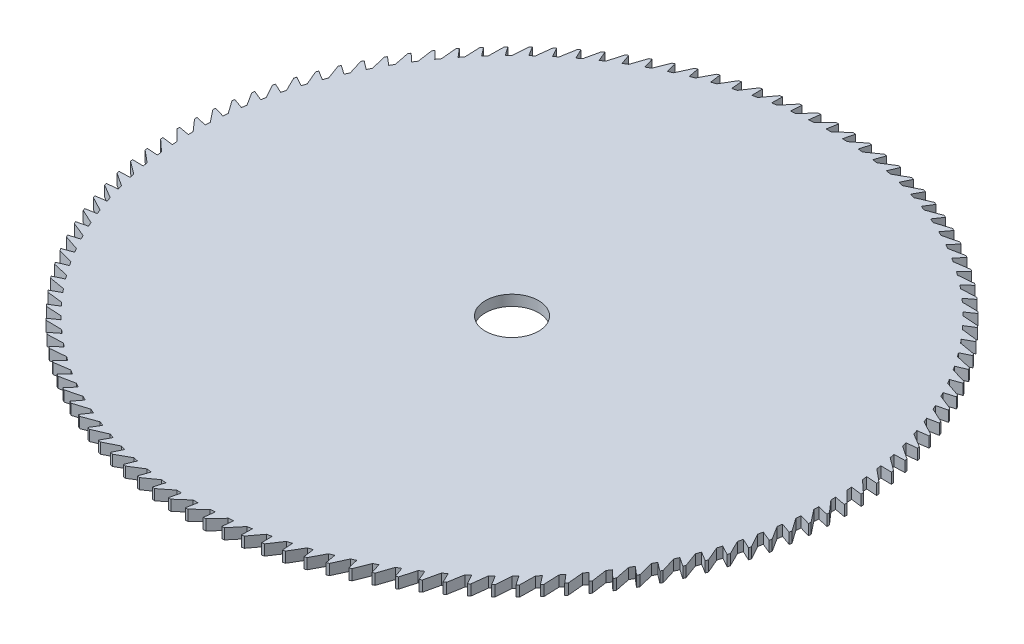
from build123d import *

# Parameters (mm, degrees)
SKETCH2_R           = 150
SKETCH2_R_2         = 12.5
BOSS_EXTRUDE1_DEPTH = 5
BOSS_EXTRUDE2_DEPTH = 5


with BuildPart() as part:
    # Sketch2 → Boss-Extrude1 (new body)
    with BuildSketch(Plane(origin=(0, 0, 0), x_dir=(1, 0, 0), z_dir=(0, 1, 0))):
        with Locations(Location((0, 0, 0), (0, 0, 270))):
            Circle(SKETCH2_R)
        with Locations(Location((0, 0, 0), (0, 0, 270))):
            Circle(SKETCH2_R_2, mode=Mode.SUBTRACT)
    extrude(amount=BOSS_EXTRUDE1_DEPTH)

    # Sketch3 → Boss-Extrude2 (add)
    with BuildSketch(Plane(origin=(0, 5, 0), x_dir=(1, 0, 0), z_dir=(0, 1, 0))):
        with BuildLine():
            Line((0, 150), (5.590008371, 154.899166578))
            ThreePointArc((5.590008371, 154.899166578), (6.178302205, 154.876817445), (6.76650691, 154.85223403))
            Line((6.76650691, 154.85223403), (5.590008371, 149.895803165))
            ThreePointArc((5.590008371, 149.895803165), (2.795489696, 149.973948529), (0, 150))
        make_face()
        with BuildLine():
            Line((7.850393436, 149.794430213), (13.689143463, 154.39432422))
            ThreePointArc((13.689143463, 154.39432422), (14.275461398, 154.341216795), (14.861573392, 154.285882816))
            Line((14.861573392, 154.285882816), (13.427287654, 149.397817743))
            ThreePointArc((13.427287654, 149.397817743), (10.640688583, 149.622109818), (7.850393436, 149.794430213))
        make_face()
        with BuildLine():
            Line((15.67926949, 149.178284305), (21.750757564, 153.466297751))
            ThreePointArc((21.750757564, 153.466297751), (22.333492543, 153.382577599), (22.915905334, 153.296644721))
            Line((22.915905334, 153.296644721), (21.227763675, 148.490343286))
            ThreePointArc((21.227763675, 148.490343286), (18.456722081, 148.860167305), (15.67926949, 149.178284305))
        make_face()
        with BuildLine():
            Line((23.465169756, 148.153251089), (29.752754351, 152.117630827))
            ThreePointArc((29.752754351, 152.117630827), (30.330309137, 152.003527418), (30.907426372, 151.887231178))
            Line((30.907426372, 151.887231178), (28.970055872, 147.175867121))
            ThreePointArc((28.970055872, 147.175867121), (26.222166987, 147.69020942), (23.465169756, 148.153251089))
        make_face()
        with BuildLine():
            Line((31.186753623, 146.72214011), (37.673200906, 150.352020051))
            ThreePointArc((37.673200906, 150.352020051), (38.243992462, 150.207846135), (38.814232304, 150.061505293))
            Line((38.814232304, 150.061505293), (36.632943159, 145.457992134))
            ThreePointArc((36.632943159, 145.457992134), (33.915738757, 146.115442937), (31.186753623, 146.72214011))
        make_face()
        with BuildLine():
            Line((38.822856765, 144.888873943), (45.490387836, 148.174304839))
            ThreePointArc((45.490387836, 148.174304839), (46.052851662, 148.000455586), (46.614651122, 147.824471251))
            Line((46.614651122, 147.824471251), (44.195422095, 143.3414269))
            ThreePointArc((44.195422095, 143.3414269), (41.516349843, 144.140184181), (38.822856765, 144.888873943))
        make_face()
        with BuildLine():
            Line((46.352549156, 142.658477444), (53.182888775, 145.590454157))
            ThreePointArc((53.182888775, 145.590454157), (53.735483197, 145.387406076), (54.287302422, 145.18226061))
            Line((54.287302422, 145.18226061), (51.636764451, 140.83197278))
            ThreePointArc((51.636764451, 140.83197278), (49.003167501, 141.769847199), (46.352549156, 142.658477444))
        make_face()
        with BuildLine():
            Line((53.755192432, 140.037063975), (60.729619112, 142.60755016))
            ThreePointArc((60.729619112, 142.60755016), (61.270829508, 142.375859792), (61.811155999, 142.142115483))
            Line((61.811155999, 142.142115483), (58.936574025, 137.936508011))
            ThreePointArc((58.936574025, 137.936508011), (56.355670883, 139.010928921), (53.755192432, 140.037063975))
        make_face()
        with BuildLine():
            Line((61.010496461, 137.031818646), (68.109893785, 139.23376878))
            ThreePointArc((68.109893785, 139.23376878), (68.638236733, 138.974071172), (69.165589494, 138.712368698))
            Line((69.165589494, 138.712368698), (66.074842546, 134.662968861))
            ThreePointArc((66.074842546, 134.662968861), (63.553707287, 135.870991348), (61.010496461, 137.031818646))
        make_face()
        with BuildLine():
            Line((68.098574961, 133.650978628), (75.303483973, 135.478357318))
            ThreePointArc((75.303483973, 135.478357318), (75.817511323, 135.191364283), (76.330444916, 134.902420953))
            Line((76.330444916, 134.902420953), (73.032004517, 131.020327874))
            ThreePointArc((73.032004517, 131.020327874), (70.577547398, 132.358640833), (68.098574961, 133.650978628))
        make_face()
        with BuildLine():
            Line((75, 129.903810568), (82.290672546, 131.351609096))
            ThreePointArc((82.290672546, 131.351609096), (82.788975384, 131.038107262), (83.286083894, 130.722715048))
            Line((83.286083894, 130.722715048), (79.788990839, 127.018569276))
            ThreePointArc((79.788990839, 127.018569276), (77.407939358, 128.483504484), (75, 129.903810568))
        make_face()
        with BuildLine():
            Line((81.695855252, 125.800585192), (89.052308105, 126.864835243))
            ThreePointArc((89.052308105, 126.864835243), (89.533520619, 126.525683897), (90.013441506, 126.184707268))
            Line((90.013441506, 126.184707268), (86.327281084, 122.668661608))
            ThreePointArc((86.327281084, 122.668661608), (84.026161536, 124.256203779), (81.695855252, 125.800585192))
        make_face()
        with BuildLine():
            Line((88.167787844, 121.352549156), (95.569857478, 122.030333695))
            ThreePointArc((95.569857478, 122.030333695), (96.032660697, 121.666462427), (96.49407853, 121.300835976))
            Line((96.49407853, 121.300835976), (92.628954252, 117.982527665))
            ThreePointArc((92.628954252, 117.982527665), (90.414073845, 119.688325457), (88.167787844, 121.352549156))
        make_face()
        with BuildLine():
            Line((94.398058657, 116.571894219), (101.825456514, 116.861355485))
            ThreePointArc((101.825456514, 116.861355485), (102.268581926, 116.473761641), (102.710231993, 116.084487525))
            Line((102.710231993, 116.084487525), (98.676737895, 112.973011815))
            ThreePointArc((98.676737895, 112.973011815), (96.554167463, 114.792389754), (94.398058657, 116.571894219))
        make_face()
        with BuildLine():
            Line((100.369590954, 111.471723822), (107.801959052, 111.372068422))
            ThreePointArc((107.801959052, 111.372068422), (108.224192082, 110.96181437), (108.64486385, 110.549959562))
            Line((108.64486385, 110.549959562), (104.454055458, 107.653844792))
            ThreePointArc((104.454055458, 107.653844792), (102.42961282, 109.58181609), (100.369590954, 111.471723822))
        make_face()
        with BuildLine():
            Line((106.066017178, 106.066017178), (113.482983913, 105.577518261))
            ThreePointArc((113.482983913, 105.577518261), (113.883167249, 105.145728478), (114.281707686, 104.712421844))
            Line((114.281707686, 104.712421844), (109.945071715, 102.039606063))
            ThreePointArc((109.945071715, 102.039606063), (108.024305727, 104.070886285), (106.066017178, 106.066017178))
        make_face()
        with BuildLine():
            Line((111.471723822, 100.369590954), (118.852959804, 99.493587461))
            ThreePointArc((118.852959804, 99.493587461), (119.229996571, 99.041445454), (119.605313305, 98.587874656))
            Line((119.605313305, 98.587874656), (115.134736174, 96.145683867))
            ThreePointArc((115.134736174, 96.145683867), (113.322911521, 98.274705415), (111.471723822, 100.369590954))
        make_face()
        with BuildLine():
            Line((116.571894219, 94.398058657), (123.897167993, 93.136951654))
            ThreePointArc((123.897167993, 93.136951654), (124.25002476, 92.665696711), (124.601089074, 92.193104957))
            Line((124.601089074, 92.193104957), (120.008824323, 89.988233034))
            ThreePointArc((120.008824323, 89.988233034), (118.310907092, 92.209160408), (116.571894219, 94.398058657))
        make_face()
        with BuildLine():
            Line((121.352549156, 88.167787844), (128.601782656, 86.525033936))
            ThreePointArc((128.601782656, 86.525033936), (128.929492268, 86.035957736), (129.255341919, 85.545640365))
            Line((129.255341919, 85.545640365), (124.553976627, 83.58413071))
            ThreePointArc((124.553976627, 83.58413071), (122.97462069, 85.890876501), (121.352549156, 88.167787844))
        make_face()
        with BuildLine():
            Line((125.800585192, 81.695855252), (132.953908773, 79.675957114))
            ThreePointArc((132.953908773, 79.675957114), (133.255572999, 79.17040018), (133.555314856, 78.663701119))
            Line((133.555314856, 78.663701119), (128.757735138, 76.950930093))
            ThreePointArc((128.757735138, 76.950930093), (127.3012694, 79.337171673), (125.800585192, 81.695855252))
        make_face()
        with BuildLine():
            Line((129.903810568, 75), (136.941617467, 72.608494032))
            ThreePointArc((136.941617467, 72.608494032), (137.216409467, 72.08784206), (137.489221958, 71.566150136))
            Line((137.489221958, 71.566150136), (132.608577647, 70.106812326))
            ThreePointArc((132.608577647, 70.106812326), (131.27899418, 72.566009171), (129.903810568, 75))
        make_face()
        with BuildLine():
            Line((133.650978628, 68.098574961), (140.553978706, 65.342016115))
            ThreePointArc((140.553978706, 65.342016115), (140.801145295, 64.807696177), (141.04628066, 64.27244131))
            Line((141.04628066, 64.27244131), (136.095949262, 63.070536659))
            ThreePointArc((136.095949262, 63.070536659), (134.896892362, 65.595948283), (133.650978628, 68.098574961))
        make_face()
        with BuildLine():
            Line((137.031818646, 61.010496461), (143.781091259, 57.896440273))
            ThreePointArc((143.781091259, 57.896440273), (143.99995497, 57.349916902), (144.21674131, 56.802566191))
            Line((144.21674131, 56.802566191), (139.210291341, 55.861389035))
            ThreePointArc((139.210291341, 55.861389035), (138.145047538, 58.446093459), (137.031818646, 61.010496461))
        make_face()
        with BuildLine():
            Line((140.037063975, 53.755192432), (146.614109835, 50.292174313))
            ThreePointArc((146.614109835, 50.292174313), (146.804070778, 49.734945492), (146.991913897, 49.176999185))
            Line((146.991913897, 49.176999185), (141.943067687, 48.499129226))
            ThreePointArc((141.943067687, 48.499129226), (141.014556742, 51.136041957), (140.037063975, 53.755192432))
        make_face()
        with BuildLine():
            Line((142.658477444, 46.352549156), (149.045269328, 42.550060999))
            ThreePointArc((149.045269328, 42.550060999), (149.205806832, 41.983654053), (149.364191865, 41.416641443))
            Line((149.364191865, 41.416641443), (144.286787951, 41.003936676))
            ThreePointArc((144.286787951, 41.003936676), (143.497554847, 43.685830117), (142.658477444, 46.352549156))
        make_face()
        with BuildLine():
            Line((144.888873943, 38.822856765), (151.067906097, 34.691320926))
            ThreePointArc((151.067906097, 34.691320926), (151.198580141, 34.117288337), (151.327072966, 33.542763566))
            Line((151.327072966, 33.542763566), (146.235028158, 33.396355185))
            ThreePointArc((146.235028158, 33.396355185), (145.587236128, 36.115878454), (144.888873943, 38.822856765))
        make_face()
        with BuildLine():
            Line((146.72214011, 31.186753623), (152.676476236, 26.737494353))
            ThreePointArc((152.676476236, 26.737494353), (152.776928651, 26.157409505), (152.875177078, 25.576947305))
            Line((152.875177078, 25.576947305), (147.782448318, 25.697236606))
            ThreePointArc((147.782448318, 25.697236606), (147.277872916, 28.446935678), (146.72214011, 31.186753623))
        make_face()
        with BuildLine():
            Line((148.153251089, 23.465169756), (153.866570766, 18.710382167))
            ThreePointArc((153.866570766, 18.710382167), (153.936526219, 18.125835031), (154.004260956, 17.541026409))
            Line((154.004260956, 17.541026409), (148.924807059, 17.927683688))
            ThreePointArc((148.924807059, 17.927683688), (148.56483129, 20.700021829), (148.153251089, 23.465169756))
        make_face()
        with BuildLine():
            Line((149.178284305, 15.67926949), (154.63492772, 10.631986123))
            ThreePointArc((154.63492772, 10.631986123), (154.674194469, 10.044578904), (154.711229859, 9.45702678))
            Line((154.711229859, 9.45702678), (149.658973256, 10.108992235))
            ThreePointArc((149.658973256, 10.108992235), (149.444583789, 12.896370659), (149.178284305, 15.67926949))
        make_face()
        with BuildLine():
            Line((149.794430213, 7.850393436), (154.979441087, 2.524448545))
            ThreePointArc((154.979441087, 2.524448545), (154.987911503, 1.935791284), (154.994146035, 1.347106097))
            Line((154.994146035, 1.347106097), (149.98293461, 2.262592736))
            ThreePointArc((149.98293461, 2.262592736), (149.914719071, 5.057371433), (149.794430213, 7.850393436))
        make_face()
        with BuildLine():
            Line((150, 0), (154.899166578, -5.590008371))
            ThreePointArc((154.899166578, -5.590008371), (154.876817445, -6.178302205), (154.85223403, -6.76650691))
            Line((154.85223403, -6.76650691), (149.895803165, -5.590008371))
            ThreePointArc((149.895803165, -5.590008371), (149.973948529, -2.795489696), (150, 0))
        make_face()
        with BuildLine():
            Line((149.794430213, -7.850393436), (154.39432422, -13.689143463))
            ThreePointArc((154.39432422, -13.689143463), (154.341216795, -14.275461398), (154.285882816, -14.861573392))
            Line((154.285882816, -14.861573392), (149.397817743, -13.427287654))
            ThreePointArc((149.397817743, -13.427287654), (149.622109818, -10.640688583), (149.794430213, -7.850393436))
        make_face()
        with BuildLine():
            Line((149.178284305, -15.67926949), (153.466297751, -21.750757564))
            ThreePointArc((153.466297751, -21.750757564), (153.382577599, -22.333492543), (153.296644721, -22.915905334))
            Line((153.296644721, -22.915905334), (148.490343286, -21.227763675))
            ThreePointArc((148.490343286, -21.227763675), (148.860167305, -18.456722081), (149.178284305, -15.67926949))
        make_face()
        with BuildLine():
            Line((148.153251089, -23.465169756), (152.117630827, -29.752754351))
            ThreePointArc((152.117630827, -29.752754351), (152.003527418, -30.330309137), (151.887231178, -30.907426372))
            Line((151.887231178, -30.907426372), (147.175867121, -28.970055872))
            ThreePointArc((147.175867121, -28.970055872), (147.69020942, -26.222166987), (148.153251089, -23.465169756))
        make_face()
        with BuildLine():
            Line((146.72214011, -31.186753623), (150.352020051, -37.673200906))
            ThreePointArc((150.352020051, -37.673200906), (150.207846135, -38.243992462), (150.061505293, -38.814232304))
            Line((150.061505293, -38.814232304), (145.457992134, -36.632943159))
            ThreePointArc((145.457992134, -36.632943159), (146.115442937, -33.915738757), (146.72214011, -31.186753623))
        make_face()
        with BuildLine():
            Line((144.888873943, -38.822856765), (148.174304839, -45.490387836))
            ThreePointArc((148.174304839, -45.490387836), (148.000455586, -46.052851662), (147.824471251, -46.614651122))
            Line((147.824471251, -46.614651122), (143.3414269, -44.195422095))
            ThreePointArc((143.3414269, -44.195422095), (144.140184181, -41.516349843), (144.888873943, -38.822856765))
        make_face()
        with BuildLine():
            Line((142.658477444, -46.352549156), (145.590454157, -53.182888775))
            ThreePointArc((145.590454157, -53.182888775), (145.387406076, -53.735483197), (145.18226061, -54.287302422))
            Line((145.18226061, -54.287302422), (140.83197278, -51.636764451))
            ThreePointArc((140.83197278, -51.636764451), (141.769847199, -49.003167501), (142.658477444, -46.352549156))
        make_face()
        with BuildLine():
            Line((140.037063975, -53.755192432), (142.60755016, -60.729619112))
            ThreePointArc((142.60755016, -60.729619112), (142.375859792, -61.270829508), (142.142115483, -61.811155999))
            Line((142.142115483, -61.811155999), (137.936508011, -58.936574025))
            ThreePointArc((137.936508011, -58.936574025), (139.010928921, -56.355670883), (140.037063975, -53.755192432))
        make_face()
        with BuildLine():
            Line((137.031818646, -61.010496461), (139.23376878, -68.109893785))
            ThreePointArc((139.23376878, -68.109893785), (138.974071172, -68.638236733), (138.712368698, -69.165589494))
            Line((138.712368698, -69.165589494), (134.662968861, -66.074842546))
            ThreePointArc((134.662968861, -66.074842546), (135.870991348, -63.553707287), (137.031818646, -61.010496461))
        make_face()
        with BuildLine():
            Line((133.650978628, -68.098574961), (135.478357318, -75.303483973))
            ThreePointArc((135.478357318, -75.303483973), (135.191364283, -75.817511323), (134.902420953, -76.330444916))
            Line((134.902420953, -76.330444916), (131.020327874, -73.032004517))
            ThreePointArc((131.020327874, -73.032004517), (132.358640833, -70.577547398), (133.650978628, -68.098574961))
        make_face()
        with BuildLine():
            Line((129.903810568, -75), (131.351609096, -82.290672546))
            ThreePointArc((131.351609096, -82.290672546), (131.038107262, -82.788975384), (130.722715048, -83.286083894))
            Line((130.722715048, -83.286083894), (127.018569276, -79.788990839))
            ThreePointArc((127.018569276, -79.788990839), (128.483504484, -77.407939358), (129.903810568, -75))
        make_face()
        with BuildLine():
            Line((125.800585192, -81.695855252), (126.864835243, -89.052308105))
            ThreePointArc((126.864835243, -89.052308105), (126.525683897, -89.533520619), (126.184707268, -90.013441506))
            Line((126.184707268, -90.013441506), (122.668661608, -86.327281084))
            ThreePointArc((122.668661608, -86.327281084), (124.256203779, -84.026161536), (125.800585192, -81.695855252))
        make_face()
        with BuildLine():
            Line((121.352549156, -88.167787844), (122.030333695, -95.569857478))
            ThreePointArc((122.030333695, -95.569857478), (121.666462427, -96.032660697), (121.300835976, -96.49407853))
            Line((121.300835976, -96.49407853), (117.982527665, -92.628954252))
            ThreePointArc((117.982527665, -92.628954252), (119.688325457, -90.414073845), (121.352549156, -88.167787844))
        make_face()
        with BuildLine():
            Line((116.571894219, -94.398058657), (116.861355485, -101.825456514))
            ThreePointArc((116.861355485, -101.825456514), (116.473761641, -102.268581926), (116.084487525, -102.710231993))
            Line((116.084487525, -102.710231993), (112.973011815, -98.676737895))
            ThreePointArc((112.973011815, -98.676737895), (114.792389754, -96.554167463), (116.571894219, -94.398058657))
        make_face()
        with BuildLine():
            Line((111.471723822, -100.369590954), (111.372068422, -107.801959052))
            ThreePointArc((111.372068422, -107.801959052), (110.96181437, -108.224192082), (110.549959562, -108.64486385))
            Line((110.549959562, -108.64486385), (107.653844792, -104.454055458))
            ThreePointArc((107.653844792, -104.454055458), (109.58181609, -102.42961282), (111.471723822, -100.369590954))
        make_face()
        with BuildLine():
            Line((106.066017178, -106.066017178), (105.577518261, -113.482983913))
            ThreePointArc((105.577518261, -113.482983913), (105.145728478, -113.883167249), (104.712421844, -114.281707686))
            Line((104.712421844, -114.281707686), (102.039606063, -109.945071715))
            ThreePointArc((102.039606063, -109.945071715), (104.070886285, -108.024305727), (106.066017178, -106.066017178))
        make_face()
        with BuildLine():
            Line((100.369590954, -111.471723822), (99.493587461, -118.852959804))
            ThreePointArc((99.493587461, -118.852959804), (99.041445454, -119.229996571), (98.587874656, -119.605313305))
            Line((98.587874656, -119.605313305), (96.145683867, -115.134736174))
            ThreePointArc((96.145683867, -115.134736174), (98.274705415, -113.322911521), (100.369590954, -111.471723822))
        make_face()
        with BuildLine():
            Line((94.398058657, -116.571894219), (93.136951654, -123.897167993))
            ThreePointArc((93.136951654, -123.897167993), (92.665696711, -124.25002476), (92.193104957, -124.601089074))
            Line((92.193104957, -124.601089074), (89.988233034, -120.008824323))
            ThreePointArc((89.988233034, -120.008824323), (92.209160408, -118.310907092), (94.398058657, -116.571894219))
        make_face()
        with BuildLine():
            Line((88.167787844, -121.352549156), (86.525033936, -128.601782656))
            ThreePointArc((86.525033936, -128.601782656), (86.035957736, -128.929492268), (85.545640365, -129.255341919))
            Line((85.545640365, -129.255341919), (83.58413071, -124.553976627))
            ThreePointArc((83.58413071, -124.553976627), (85.890876501, -122.97462069), (88.167787844, -121.352549156))
        make_face()
        with BuildLine():
            Line((81.695855252, -125.800585192), (79.675957114, -132.953908773))
            ThreePointArc((79.675957114, -132.953908773), (79.17040018, -133.255572999), (78.663701119, -133.555314856))
            Line((78.663701119, -133.555314856), (76.950930093, -128.757735138))
            ThreePointArc((76.950930093, -128.757735138), (79.337171673, -127.3012694), (81.695855252, -125.800585192))
        make_face()
        with BuildLine():
            Line((75, -129.903810568), (72.608494032, -136.941617467))
            ThreePointArc((72.608494032, -136.941617467), (72.08784206, -137.216409467), (71.566150136, -137.489221958))
            Line((71.566150136, -137.489221958), (70.106812326, -132.608577647))
            ThreePointArc((70.106812326, -132.608577647), (72.566009171, -131.27899418), (75, -129.903810568))
        make_face()
        with BuildLine():
            Line((68.098574961, -133.650978628), (65.342016115, -140.553978706))
            ThreePointArc((65.342016115, -140.553978706), (64.807696177, -140.801145295), (64.27244131, -141.04628066))
            Line((64.27244131, -141.04628066), (63.070536659, -136.095949262))
            ThreePointArc((63.070536659, -136.095949262), (65.595948283, -134.896892362), (68.098574961, -133.650978628))
        make_face()
        with BuildLine():
            Line((61.010496461, -137.031818646), (57.896440273, -143.781091259))
            ThreePointArc((57.896440273, -143.781091259), (57.349916902, -143.99995497), (56.802566191, -144.21674131))
            Line((56.802566191, -144.21674131), (55.861389035, -139.210291341))
            ThreePointArc((55.861389035, -139.210291341), (58.446093459, -138.145047538), (61.010496461, -137.031818646))
        make_face()
        with BuildLine():
            Line((53.755192432, -140.037063975), (50.292174313, -146.614109835))
            ThreePointArc((50.292174313, -146.614109835), (49.734945492, -146.804070778), (49.176999185, -146.991913897))
            Line((49.176999185, -146.991913897), (48.499129226, -141.943067687))
            ThreePointArc((48.499129226, -141.943067687), (51.136041957, -141.014556742), (53.755192432, -140.037063975))
        make_face()
        with BuildLine():
            Line((46.352549156, -142.658477444), (42.550060999, -149.045269328))
            ThreePointArc((42.550060999, -149.045269328), (41.983654053, -149.205806832), (41.416641443, -149.364191865))
            Line((41.416641443, -149.364191865), (41.003936676, -144.286787951))
            ThreePointArc((41.003936676, -144.286787951), (43.685830117, -143.497554847), (46.352549156, -142.658477444))
        make_face()
        with BuildLine():
            Line((38.822856765, -144.888873943), (34.691320926, -151.067906097))
            ThreePointArc((34.691320926, -151.067906097), (34.117288337, -151.198580141), (33.542763566, -151.327072966))
            Line((33.542763566, -151.327072966), (33.396355185, -146.235028158))
            ThreePointArc((33.396355185, -146.235028158), (36.115878454, -145.587236128), (38.822856765, -144.888873943))
        make_face()
        with BuildLine():
            Line((31.186753623, -146.72214011), (26.737494353, -152.676476236))
            ThreePointArc((26.737494353, -152.676476236), (26.157409505, -152.776928651), (25.576947305, -152.875177078))
            Line((25.576947305, -152.875177078), (25.697236606, -147.782448318))
            ThreePointArc((25.697236606, -147.782448318), (28.446935678, -147.277872916), (31.186753623, -146.72214011))
        make_face()
        with BuildLine():
            Line((23.465169756, -148.153251089), (18.710382167, -153.866570766))
            ThreePointArc((18.710382167, -153.866570766), (18.125835031, -153.936526219), (17.541026409, -154.004260956))
            Line((17.541026409, -154.004260956), (17.927683688, -148.924807059))
            ThreePointArc((17.927683688, -148.924807059), (20.700021829, -148.56483129), (23.465169756, -148.153251089))
        make_face()
        with BuildLine():
            Line((15.67926949, -149.178284305), (10.631986123, -154.63492772))
            ThreePointArc((10.631986123, -154.63492772), (10.044578904, -154.674194469), (9.45702678, -154.711229859))
            Line((9.45702678, -154.711229859), (10.108992235, -149.658973256))
            ThreePointArc((10.108992235, -149.658973256), (12.896370659, -149.444583789), (15.67926949, -149.178284305))
        make_face()
        with BuildLine():
            Line((7.850393436, -149.794430213), (2.524448545, -154.979441087))
            ThreePointArc((2.524448545, -154.979441087), (1.935791284, -154.987911503), (1.347106097, -154.994146035))
            Line((1.347106097, -154.994146035), (2.262592736, -149.98293461))
            ThreePointArc((2.262592736, -149.98293461), (5.057371433, -149.914719071), (7.850393436, -149.794430213))
        make_face()
        with BuildLine():
            Line((0, -150), (-5.590008371, -154.899166578))
            ThreePointArc((-5.590008371, -154.899166578), (-6.178302205, -154.876817445), (-6.76650691, -154.85223403))
            Line((-6.76650691, -154.85223403), (-5.590008371, -149.895803165))
            ThreePointArc((-5.590008371, -149.895803165), (-2.795489696, -149.973948529), (0, -150))
        make_face()
        with BuildLine():
            Line((-7.850393436, -149.794430213), (-13.689143463, -154.39432422))
            ThreePointArc((-13.689143463, -154.39432422), (-14.275461398, -154.341216795), (-14.861573392, -154.285882816))
            Line((-14.861573392, -154.285882816), (-13.427287654, -149.397817743))
            ThreePointArc((-13.427287654, -149.397817743), (-10.640688583, -149.622109818), (-7.850393436, -149.794430213))
        make_face()
        with BuildLine():
            Line((-15.67926949, -149.178284305), (-21.750757564, -153.466297751))
            ThreePointArc((-21.750757564, -153.466297751), (-22.333492543, -153.382577599), (-22.915905334, -153.296644721))
            Line((-22.915905334, -153.296644721), (-21.227763675, -148.490343286))
            ThreePointArc((-21.227763675, -148.490343286), (-18.456722081, -148.860167305), (-15.67926949, -149.178284305))
        make_face()
        with BuildLine():
            Line((-23.465169756, -148.153251089), (-29.752754351, -152.117630827))
            ThreePointArc((-29.752754351, -152.117630827), (-30.330309137, -152.003527418), (-30.907426372, -151.887231178))
            Line((-30.907426372, -151.887231178), (-28.970055872, -147.175867121))
            ThreePointArc((-28.970055872, -147.175867121), (-26.222166987, -147.69020942), (-23.465169756, -148.153251089))
        make_face()
        with BuildLine():
            Line((-31.186753623, -146.72214011), (-37.673200906, -150.352020051))
            ThreePointArc((-37.673200906, -150.352020051), (-38.243992462, -150.207846135), (-38.814232304, -150.061505293))
            Line((-38.814232304, -150.061505293), (-36.632943159, -145.457992134))
            ThreePointArc((-36.632943159, -145.457992134), (-33.915738757, -146.115442937), (-31.186753623, -146.72214011))
        make_face()
        with BuildLine():
            Line((-38.822856765, -144.888873943), (-45.490387836, -148.174304839))
            ThreePointArc((-45.490387836, -148.174304839), (-46.052851662, -148.000455586), (-46.614651122, -147.824471251))
            Line((-46.614651122, -147.824471251), (-44.195422095, -143.3414269))
            ThreePointArc((-44.195422095, -143.3414269), (-41.516349843, -144.140184181), (-38.822856765, -144.888873943))
        make_face()
        with BuildLine():
            Line((-46.352549156, -142.658477444), (-53.182888775, -145.590454157))
            ThreePointArc((-53.182888775, -145.590454157), (-53.735483197, -145.387406076), (-54.287302422, -145.18226061))
            Line((-54.287302422, -145.18226061), (-51.636764451, -140.83197278))
            ThreePointArc((-51.636764451, -140.83197278), (-49.003167501, -141.769847199), (-46.352549156, -142.658477444))
        make_face()
        with BuildLine():
            Line((-53.755192432, -140.037063975), (-60.729619112, -142.60755016))
            ThreePointArc((-60.729619112, -142.60755016), (-61.270829508, -142.375859792), (-61.811155999, -142.142115483))
            Line((-61.811155999, -142.142115483), (-58.936574025, -137.936508011))
            ThreePointArc((-58.936574025, -137.936508011), (-56.355670883, -139.010928921), (-53.755192432, -140.037063975))
        make_face()
        with BuildLine():
            Line((-61.010496461, -137.031818646), (-68.109893785, -139.23376878))
            ThreePointArc((-68.109893785, -139.23376878), (-68.638236733, -138.974071172), (-69.165589494, -138.712368698))
            Line((-69.165589494, -138.712368698), (-66.074842546, -134.662968861))
            ThreePointArc((-66.074842546, -134.662968861), (-63.553707287, -135.870991348), (-61.010496461, -137.031818646))
        make_face()
        with BuildLine():
            Line((-68.098574961, -133.650978628), (-75.303483973, -135.478357318))
            ThreePointArc((-75.303483973, -135.478357318), (-75.817511323, -135.191364283), (-76.330444916, -134.902420953))
            Line((-76.330444916, -134.902420953), (-73.032004517, -131.020327874))
            ThreePointArc((-73.032004517, -131.020327874), (-70.577547398, -132.358640833), (-68.098574961, -133.650978628))
        make_face()
        with BuildLine():
            Line((-75, -129.903810568), (-82.290672546, -131.351609096))
            ThreePointArc((-82.290672546, -131.351609096), (-82.788975384, -131.038107262), (-83.286083894, -130.722715048))
            Line((-83.286083894, -130.722715048), (-79.788990839, -127.018569276))
            ThreePointArc((-79.788990839, -127.018569276), (-77.407939358, -128.483504484), (-75, -129.903810568))
        make_face()
        with BuildLine():
            Line((-81.695855252, -125.800585192), (-89.052308105, -126.864835243))
            ThreePointArc((-89.052308105, -126.864835243), (-89.533520619, -126.525683897), (-90.013441506, -126.184707268))
            Line((-90.013441506, -126.184707268), (-86.327281084, -122.668661608))
            ThreePointArc((-86.327281084, -122.668661608), (-84.026161536, -124.256203779), (-81.695855252, -125.800585192))
        make_face()
        with BuildLine():
            Line((-88.167787844, -121.352549156), (-95.569857478, -122.030333695))
            ThreePointArc((-95.569857478, -122.030333695), (-96.032660697, -121.666462427), (-96.49407853, -121.300835976))
            Line((-96.49407853, -121.300835976), (-92.628954252, -117.982527665))
            ThreePointArc((-92.628954252, -117.982527665), (-90.414073845, -119.688325457), (-88.167787844, -121.352549156))
        make_face()
        with BuildLine():
            Line((-94.398058657, -116.571894219), (-101.825456514, -116.861355485))
            ThreePointArc((-101.825456514, -116.861355485), (-102.268581926, -116.473761641), (-102.710231993, -116.084487525))
            Line((-102.710231993, -116.084487525), (-98.676737895, -112.973011815))
            ThreePointArc((-98.676737895, -112.973011815), (-96.554167463, -114.792389754), (-94.398058657, -116.571894219))
        make_face()
        with BuildLine():
            Line((-100.369590954, -111.471723822), (-107.801959052, -111.372068422))
            ThreePointArc((-107.801959052, -111.372068422), (-108.224192082, -110.96181437), (-108.64486385, -110.549959562))
            Line((-108.64486385, -110.549959562), (-104.454055458, -107.653844792))
            ThreePointArc((-104.454055458, -107.653844792), (-102.42961282, -109.58181609), (-100.369590954, -111.471723822))
        make_face()
        with BuildLine():
            Line((-106.066017178, -106.066017178), (-113.482983913, -105.577518261))
            ThreePointArc((-113.482983913, -105.577518261), (-113.883167249, -105.145728478), (-114.281707686, -104.712421844))
            Line((-114.281707686, -104.712421844), (-109.945071715, -102.039606063))
            ThreePointArc((-109.945071715, -102.039606063), (-108.024305727, -104.070886285), (-106.066017178, -106.066017178))
        make_face()
        with BuildLine():
            Line((-111.471723822, -100.369590954), (-118.852959804, -99.493587461))
            ThreePointArc((-118.852959804, -99.493587461), (-119.229996571, -99.041445454), (-119.605313305, -98.587874656))
            Line((-119.605313305, -98.587874656), (-115.134736174, -96.145683867))
            ThreePointArc((-115.134736174, -96.145683867), (-113.322911521, -98.274705415), (-111.471723822, -100.369590954))
        make_face()
        with BuildLine():
            Line((-116.571894219, -94.398058657), (-123.897167993, -93.136951654))
            ThreePointArc((-123.897167993, -93.136951654), (-124.25002476, -92.665696711), (-124.601089074, -92.193104957))
            Line((-124.601089074, -92.193104957), (-120.008824323, -89.988233034))
            ThreePointArc((-120.008824323, -89.988233034), (-118.310907092, -92.209160408), (-116.571894219, -94.398058657))
        make_face()
        with BuildLine():
            Line((-121.352549156, -88.167787844), (-128.601782656, -86.525033936))
            ThreePointArc((-128.601782656, -86.525033936), (-128.929492268, -86.035957736), (-129.255341919, -85.545640365))
            Line((-129.255341919, -85.545640365), (-124.553976627, -83.58413071))
            ThreePointArc((-124.553976627, -83.58413071), (-122.97462069, -85.890876501), (-121.352549156, -88.167787844))
        make_face()
        with BuildLine():
            Line((-125.800585192, -81.695855252), (-132.953908773, -79.675957114))
            ThreePointArc((-132.953908773, -79.675957114), (-133.255572999, -79.17040018), (-133.555314856, -78.663701119))
            Line((-133.555314856, -78.663701119), (-128.757735138, -76.950930093))
            ThreePointArc((-128.757735138, -76.950930093), (-127.3012694, -79.337171673), (-125.800585192, -81.695855252))
        make_face()
        with BuildLine():
            Line((-129.903810568, -75), (-136.941617467, -72.608494032))
            ThreePointArc((-136.941617467, -72.608494032), (-137.216409467, -72.08784206), (-137.489221958, -71.566150136))
            Line((-137.489221958, -71.566150136), (-132.608577647, -70.106812326))
            ThreePointArc((-132.608577647, -70.106812326), (-131.27899418, -72.566009171), (-129.903810568, -75))
        make_face()
        with BuildLine():
            Line((-133.650978628, -68.098574961), (-140.553978706, -65.342016115))
            ThreePointArc((-140.553978706, -65.342016115), (-140.801145295, -64.807696177), (-141.04628066, -64.27244131))
            Line((-141.04628066, -64.27244131), (-136.095949262, -63.070536659))
            ThreePointArc((-136.095949262, -63.070536659), (-134.896892362, -65.595948283), (-133.650978628, -68.098574961))
        make_face()
        with BuildLine():
            Line((-137.031818646, -61.010496461), (-143.781091259, -57.896440273))
            ThreePointArc((-143.781091259, -57.896440273), (-143.99995497, -57.349916902), (-144.21674131, -56.802566191))
            Line((-144.21674131, -56.802566191), (-139.210291341, -55.861389035))
            ThreePointArc((-139.210291341, -55.861389035), (-138.145047538, -58.446093459), (-137.031818646, -61.010496461))
        make_face()
        with BuildLine():
            Line((-140.037063975, -53.755192432), (-146.614109835, -50.292174313))
            ThreePointArc((-146.614109835, -50.292174313), (-146.804070778, -49.734945492), (-146.991913897, -49.176999185))
            Line((-146.991913897, -49.176999185), (-141.943067687, -48.499129226))
            ThreePointArc((-141.943067687, -48.499129226), (-141.014556742, -51.136041957), (-140.037063975, -53.755192432))
        make_face()
        with BuildLine():
            Line((-142.658477444, -46.352549156), (-149.045269328, -42.550060999))
            ThreePointArc((-149.045269328, -42.550060999), (-149.205806832, -41.983654053), (-149.364191865, -41.416641443))
            Line((-149.364191865, -41.416641443), (-144.286787951, -41.003936676))
            ThreePointArc((-144.286787951, -41.003936676), (-143.497554847, -43.685830117), (-142.658477444, -46.352549156))
        make_face()
        with BuildLine():
            Line((-144.888873943, -38.822856765), (-151.067906097, -34.691320926))
            ThreePointArc((-151.067906097, -34.691320926), (-151.198580141, -34.117288337), (-151.327072966, -33.542763566))
            Line((-151.327072966, -33.542763566), (-146.235028158, -33.396355185))
            ThreePointArc((-146.235028158, -33.396355185), (-145.587236128, -36.115878454), (-144.888873943, -38.822856765))
        make_face()
        with BuildLine():
            Line((-146.72214011, -31.186753623), (-152.676476236, -26.737494353))
            ThreePointArc((-152.676476236, -26.737494353), (-152.776928651, -26.157409505), (-152.875177078, -25.576947305))
            Line((-152.875177078, -25.576947305), (-147.782448318, -25.697236606))
            ThreePointArc((-147.782448318, -25.697236606), (-147.277872916, -28.446935678), (-146.72214011, -31.186753623))
        make_face()
        with BuildLine():
            Line((-148.153251089, -23.465169756), (-153.866570766, -18.710382167))
            ThreePointArc((-153.866570766, -18.710382167), (-153.936526219, -18.125835031), (-154.004260956, -17.541026409))
            Line((-154.004260956, -17.541026409), (-148.924807059, -17.927683688))
            ThreePointArc((-148.924807059, -17.927683688), (-148.56483129, -20.700021829), (-148.153251089, -23.465169756))
        make_face()
        with BuildLine():
            Line((-149.178284305, -15.67926949), (-154.63492772, -10.631986123))
            ThreePointArc((-154.63492772, -10.631986123), (-154.674194469, -10.044578904), (-154.711229859, -9.45702678))
            Line((-154.711229859, -9.45702678), (-149.658973256, -10.108992235))
            ThreePointArc((-149.658973256, -10.108992235), (-149.444583789, -12.896370659), (-149.178284305, -15.67926949))
        make_face()
        with BuildLine():
            Line((-149.794430213, -7.850393436), (-154.979441087, -2.524448545))
            ThreePointArc((-154.979441087, -2.524448545), (-154.987911503, -1.935791284), (-154.994146035, -1.347106097))
            Line((-154.994146035, -1.347106097), (-149.98293461, -2.262592736))
            ThreePointArc((-149.98293461, -2.262592736), (-149.914719071, -5.057371433), (-149.794430213, -7.850393436))
        make_face()
        with BuildLine():
            Line((-150, 0), (-154.899166578, 5.590008371))
            ThreePointArc((-154.899166578, 5.590008371), (-154.876817445, 6.178302205), (-154.85223403, 6.76650691))
            Line((-154.85223403, 6.76650691), (-149.895803165, 5.590008371))
            ThreePointArc((-149.895803165, 5.590008371), (-149.973948529, 2.795489696), (-150, 0))
        make_face()
        with BuildLine():
            Line((-149.794430213, 7.850393436), (-154.39432422, 13.689143463))
            ThreePointArc((-154.39432422, 13.689143463), (-154.341216795, 14.275461398), (-154.285882816, 14.861573392))
            Line((-154.285882816, 14.861573392), (-149.397817743, 13.427287654))
            ThreePointArc((-149.397817743, 13.427287654), (-149.622109818, 10.640688583), (-149.794430213, 7.850393436))
        make_face()
        with BuildLine():
            Line((-149.178284305, 15.67926949), (-153.466297751, 21.750757564))
            ThreePointArc((-153.466297751, 21.750757564), (-153.382577599, 22.333492543), (-153.296644721, 22.915905334))
            Line((-153.296644721, 22.915905334), (-148.490343286, 21.227763675))
            ThreePointArc((-148.490343286, 21.227763675), (-148.860167305, 18.456722081), (-149.178284305, 15.67926949))
        make_face()
        with BuildLine():
            Line((-148.153251089, 23.465169756), (-152.117630827, 29.752754351))
            ThreePointArc((-152.117630827, 29.752754351), (-152.003527418, 30.330309137), (-151.887231178, 30.907426372))
            Line((-151.887231178, 30.907426372), (-147.175867121, 28.970055872))
            ThreePointArc((-147.175867121, 28.970055872), (-147.69020942, 26.222166987), (-148.153251089, 23.465169756))
        make_face()
        with BuildLine():
            Line((-146.72214011, 31.186753623), (-150.352020051, 37.673200906))
            ThreePointArc((-150.352020051, 37.673200906), (-150.207846135, 38.243992462), (-150.061505293, 38.814232304))
            Line((-150.061505293, 38.814232304), (-145.457992134, 36.632943159))
            ThreePointArc((-145.457992134, 36.632943159), (-146.115442937, 33.915738757), (-146.72214011, 31.186753623))
        make_face()
        with BuildLine():
            Line((-144.888873943, 38.822856765), (-148.174304839, 45.490387836))
            ThreePointArc((-148.174304839, 45.490387836), (-148.000455586, 46.052851662), (-147.824471251, 46.614651122))
            Line((-147.824471251, 46.614651122), (-143.3414269, 44.195422095))
            ThreePointArc((-143.3414269, 44.195422095), (-144.140184181, 41.516349843), (-144.888873943, 38.822856765))
        make_face()
        with BuildLine():
            Line((-142.658477444, 46.352549156), (-145.590454157, 53.182888775))
            ThreePointArc((-145.590454157, 53.182888775), (-145.387406076, 53.735483197), (-145.18226061, 54.287302422))
            Line((-145.18226061, 54.287302422), (-140.83197278, 51.636764451))
            ThreePointArc((-140.83197278, 51.636764451), (-141.769847199, 49.003167501), (-142.658477444, 46.352549156))
        make_face()
        with BuildLine():
            Line((-140.037063975, 53.755192432), (-142.60755016, 60.729619112))
            ThreePointArc((-142.60755016, 60.729619112), (-142.375859792, 61.270829508), (-142.142115483, 61.811155999))
            Line((-142.142115483, 61.811155999), (-137.936508011, 58.936574025))
            ThreePointArc((-137.936508011, 58.936574025), (-139.010928921, 56.355670883), (-140.037063975, 53.755192432))
        make_face()
        with BuildLine():
            Line((-137.031818646, 61.010496461), (-139.23376878, 68.109893785))
            ThreePointArc((-139.23376878, 68.109893785), (-138.974071172, 68.638236733), (-138.712368698, 69.165589494))
            Line((-138.712368698, 69.165589494), (-134.662968861, 66.074842546))
            ThreePointArc((-134.662968861, 66.074842546), (-135.870991348, 63.553707287), (-137.031818646, 61.010496461))
        make_face()
        with BuildLine():
            Line((-133.650978628, 68.098574961), (-135.478357318, 75.303483973))
            ThreePointArc((-135.478357318, 75.303483973), (-135.191364283, 75.817511323), (-134.902420953, 76.330444916))
            Line((-134.902420953, 76.330444916), (-131.020327874, 73.032004517))
            ThreePointArc((-131.020327874, 73.032004517), (-132.358640833, 70.577547398), (-133.650978628, 68.098574961))
        make_face()
        with BuildLine():
            Line((-129.903810568, 75), (-131.351609096, 82.290672546))
            ThreePointArc((-131.351609096, 82.290672546), (-131.038107262, 82.788975384), (-130.722715048, 83.286083894))
            Line((-130.722715048, 83.286083894), (-127.018569276, 79.788990839))
            ThreePointArc((-127.018569276, 79.788990839), (-128.483504484, 77.407939358), (-129.903810568, 75))
        make_face()
        with BuildLine():
            Line((-125.800585192, 81.695855252), (-126.864835243, 89.052308105))
            ThreePointArc((-126.864835243, 89.052308105), (-126.525683897, 89.533520619), (-126.184707268, 90.013441506))
            Line((-126.184707268, 90.013441506), (-122.668661608, 86.327281084))
            ThreePointArc((-122.668661608, 86.327281084), (-124.256203779, 84.026161536), (-125.800585192, 81.695855252))
        make_face()
        with BuildLine():
            Line((-121.352549156, 88.167787844), (-122.030333695, 95.569857478))
            ThreePointArc((-122.030333695, 95.569857478), (-121.666462427, 96.032660697), (-121.300835976, 96.49407853))
            Line((-121.300835976, 96.49407853), (-117.982527665, 92.628954252))
            ThreePointArc((-117.982527665, 92.628954252), (-119.688325457, 90.414073845), (-121.352549156, 88.167787844))
        make_face()
        with BuildLine():
            Line((-116.571894219, 94.398058657), (-116.861355485, 101.825456514))
            ThreePointArc((-116.861355485, 101.825456514), (-116.473761641, 102.268581926), (-116.084487525, 102.710231993))
            Line((-116.084487525, 102.710231993), (-112.973011815, 98.676737895))
            ThreePointArc((-112.973011815, 98.676737895), (-114.792389754, 96.554167463), (-116.571894219, 94.398058657))
        make_face()
        with BuildLine():
            Line((-111.471723822, 100.369590954), (-111.372068422, 107.801959052))
            ThreePointArc((-111.372068422, 107.801959052), (-110.96181437, 108.224192082), (-110.549959562, 108.64486385))
            Line((-110.549959562, 108.64486385), (-107.653844792, 104.454055458))
            ThreePointArc((-107.653844792, 104.454055458), (-109.58181609, 102.42961282), (-111.471723822, 100.369590954))
        make_face()
        with BuildLine():
            Line((-106.066017178, 106.066017178), (-105.577518261, 113.482983913))
            ThreePointArc((-105.577518261, 113.482983913), (-105.145728478, 113.883167249), (-104.712421844, 114.281707686))
            Line((-104.712421844, 114.281707686), (-102.039606063, 109.945071715))
            ThreePointArc((-102.039606063, 109.945071715), (-104.070886285, 108.024305727), (-106.066017178, 106.066017178))
        make_face()
        with BuildLine():
            Line((-100.369590954, 111.471723822), (-99.493587461, 118.852959804))
            ThreePointArc((-99.493587461, 118.852959804), (-99.041445454, 119.229996571), (-98.587874656, 119.605313305))
            Line((-98.587874656, 119.605313305), (-96.145683867, 115.134736174))
            ThreePointArc((-96.145683867, 115.134736174), (-98.274705415, 113.322911521), (-100.369590954, 111.471723822))
        make_face()
        with BuildLine():
            Line((-94.398058657, 116.571894219), (-93.136951654, 123.897167993))
            ThreePointArc((-93.136951654, 123.897167993), (-92.665696711, 124.25002476), (-92.193104957, 124.601089074))
            Line((-92.193104957, 124.601089074), (-89.988233034, 120.008824323))
            ThreePointArc((-89.988233034, 120.008824323), (-92.209160408, 118.310907092), (-94.398058657, 116.571894219))
        make_face()
        with BuildLine():
            Line((-88.167787844, 121.352549156), (-86.525033936, 128.601782656))
            ThreePointArc((-86.525033936, 128.601782656), (-86.035957736, 128.929492268), (-85.545640365, 129.255341919))
            Line((-85.545640365, 129.255341919), (-83.58413071, 124.553976627))
            ThreePointArc((-83.58413071, 124.553976627), (-85.890876501, 122.97462069), (-88.167787844, 121.352549156))
        make_face()
        with BuildLine():
            Line((-81.695855252, 125.800585192), (-79.675957114, 132.953908773))
            ThreePointArc((-79.675957114, 132.953908773), (-79.17040018, 133.255572999), (-78.663701119, 133.555314856))
            Line((-78.663701119, 133.555314856), (-76.950930093, 128.757735138))
            ThreePointArc((-76.950930093, 128.757735138), (-79.337171673, 127.3012694), (-81.695855252, 125.800585192))
        make_face()
        with BuildLine():
            Line((-75, 129.903810568), (-72.608494032, 136.941617467))
            ThreePointArc((-72.608494032, 136.941617467), (-72.08784206, 137.216409467), (-71.566150136, 137.489221958))
            Line((-71.566150136, 137.489221958), (-70.106812326, 132.608577647))
            ThreePointArc((-70.106812326, 132.608577647), (-72.566009171, 131.27899418), (-75, 129.903810568))
        make_face()
        with BuildLine():
            Line((-68.098574961, 133.650978628), (-65.342016115, 140.553978706))
            ThreePointArc((-65.342016115, 140.553978706), (-64.807696177, 140.801145295), (-64.27244131, 141.04628066))
            Line((-64.27244131, 141.04628066), (-63.070536659, 136.095949262))
            ThreePointArc((-63.070536659, 136.095949262), (-65.595948283, 134.896892362), (-68.098574961, 133.650978628))
        make_face()
        with BuildLine():
            Line((-61.010496461, 137.031818646), (-57.896440273, 143.781091259))
            ThreePointArc((-57.896440273, 143.781091259), (-57.349916902, 143.99995497), (-56.802566191, 144.21674131))
            Line((-56.802566191, 144.21674131), (-55.861389035, 139.210291341))
            ThreePointArc((-55.861389035, 139.210291341), (-58.446093459, 138.145047538), (-61.010496461, 137.031818646))
        make_face()
        with BuildLine():
            Line((-53.755192432, 140.037063975), (-50.292174313, 146.614109835))
            ThreePointArc((-50.292174313, 146.614109835), (-49.734945492, 146.804070778), (-49.176999185, 146.991913897))
            Line((-49.176999185, 146.991913897), (-48.499129226, 141.943067687))
            ThreePointArc((-48.499129226, 141.943067687), (-51.136041957, 141.014556742), (-53.755192432, 140.037063975))
        make_face()
        with BuildLine():
            Line((-46.352549156, 142.658477444), (-42.550060999, 149.045269328))
            ThreePointArc((-42.550060999, 149.045269328), (-41.983654053, 149.205806832), (-41.416641443, 149.364191865))
            Line((-41.416641443, 149.364191865), (-41.003936676, 144.286787951))
            ThreePointArc((-41.003936676, 144.286787951), (-43.685830117, 143.497554847), (-46.352549156, 142.658477444))
        make_face()
        with BuildLine():
            Line((-38.822856765, 144.888873943), (-34.691320926, 151.067906097))
            ThreePointArc((-34.691320926, 151.067906097), (-34.117288337, 151.198580141), (-33.542763566, 151.327072966))
            Line((-33.542763566, 151.327072966), (-33.396355185, 146.235028158))
            ThreePointArc((-33.396355185, 146.235028158), (-36.115878454, 145.587236128), (-38.822856765, 144.888873943))
        make_face()
        with BuildLine():
            Line((-31.186753623, 146.72214011), (-26.737494353, 152.676476236))
            ThreePointArc((-26.737494353, 152.676476236), (-26.157409505, 152.776928651), (-25.576947305, 152.875177078))
            Line((-25.576947305, 152.875177078), (-25.697236606, 147.782448318))
            ThreePointArc((-25.697236606, 147.782448318), (-28.446935678, 147.277872916), (-31.186753623, 146.72214011))
        make_face()
        with BuildLine():
            Line((-23.465169756, 148.153251089), (-18.710382167, 153.866570766))
            ThreePointArc((-18.710382167, 153.866570766), (-18.125835031, 153.936526219), (-17.541026409, 154.004260956))
            Line((-17.541026409, 154.004260956), (-17.927683688, 148.924807059))
            ThreePointArc((-17.927683688, 148.924807059), (-20.700021829, 148.56483129), (-23.465169756, 148.153251089))
        make_face()
        with BuildLine():
            Line((-15.67926949, 149.178284305), (-10.631986123, 154.63492772))
            ThreePointArc((-10.631986123, 154.63492772), (-10.044578904, 154.674194469), (-9.45702678, 154.711229859))
            Line((-9.45702678, 154.711229859), (-10.108992235, 149.658973256))
            ThreePointArc((-10.108992235, 149.658973256), (-12.896370659, 149.444583789), (-15.67926949, 149.178284305))
        make_face()
        with BuildLine():
            Line((-7.850393436, 149.794430213), (-2.524448545, 154.979441087))
            ThreePointArc((-2.524448545, 154.979441087), (-1.935791284, 154.987911503), (-1.347106097, 154.994146035))
            Line((-1.347106097, 154.994146035), (-2.262592736, 149.98293461))
            ThreePointArc((-2.262592736, 149.98293461), (-5.057371433, 149.914719071), (-7.850393436, 149.794430213))
        make_face()
    extrude(amount=-BOSS_EXTRUDE2_DEPTH)


solid = part.part
